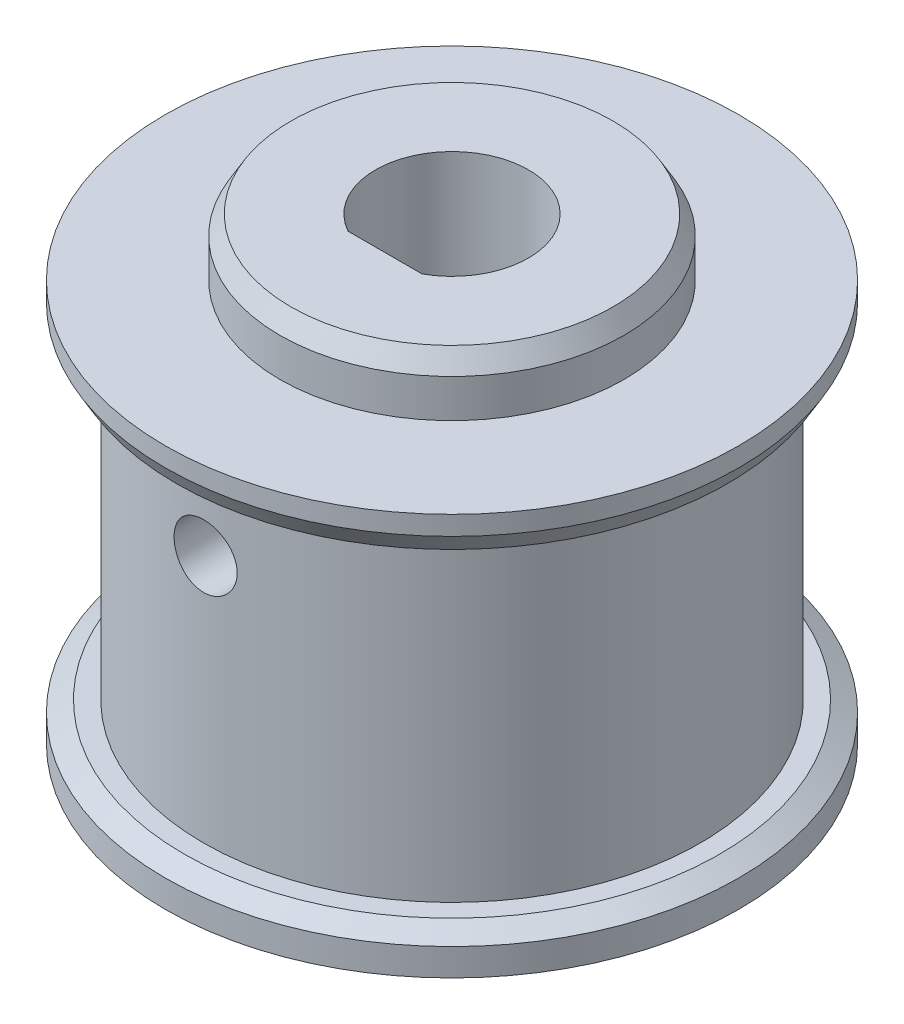
SolidWorks part; units mm, degrees
material "6061 合金"
ref_plane "前视基准面" through (0, 0, 0) normal (0, 0, 1) x (1, 0, 0)
ref_plane "上视基准面" through (0, 0, 0) normal (0, 1, 0) x (1, 0, 0)
ref_plane "右视基准面" through (0, 0, 0) normal (1, 0, 0) x (0, 0, -1)
sketch "草图1" plane through (0, 0, 0) normal (0, 0, 1) x (1, 0, 0)
  line L0 (0, 0) -> (0, 32.2299) construction
  line L1 (4, 0) -> (4, 21)
  line L2 (4, 21) -> (15, 21)
  line L3 (15, 21) -> (15, 19)
  line L4 (15, 19) -> (12.99, 19)
  line L5 (12.99, 19) -> (12.99, 2)
  line L6 (12.99, 2) -> (15, 2)
  line L7 (15, 2) -> (15, 0)
  line L8 (15, 0) -> (4, 0)
  dimension "D1" = 2
  dimension "D2" = 2
  dimension "D3" = 8
  dimension "D4" = 25.98
  dimension "D5" = 30
  dimension "D6" = 21
revolve "旋转1" add sketch "草图1" angle 360 about L0
sketch "草图5" plane through (0, 0, 0) normal (0, -1, 0) x (1, 0, 0)
  circle A0 centre (0, 0) radius 20.5663
extrude "切除-拉伸1" cut sketch "草图5" against normal blind 0.5
sketch "草图6" plane through (0, 21, 0) normal (0, 1, 0) x (1, 0, 0)
  circle A0 centre (0, 0) radius 21.5283
extrude "切除-拉伸2" cut sketch "草图6" against normal blind 0.5
sketch "草图7" plane through (0, 20.5, 0) normal (0, 1, 0) x (1, 0, 0)
  circle A0 centre (0, 0) radius 4 construction
  circle A1 centre (0, 0) radius 4
  circle A2 centre (0, 0) radius 8.5
  dimension "D1" = 17
extrude "凸台-拉伸1" add sketch "草图7" along normal blind 11
sketch "草图10" plane through (0, 20.5, 0) normal (0, 1, 0) x (1, 0, 0)
  circle A1 centre (0, 0) radius 15
  circle A2 centre (0, 0) radius 15
  dimension "D1" = 0
extrude "切除-拉伸3" cut sketch "草图10" along normal blind 15
sketch "草图11" plane through (0, 20.5, 0) normal (0, 1, 0) x (1, 0, 0)
  circle A0 centre (0, 0) radius 4 construction
  circle A1 centre (0, 0) radius 15
  circle A2 centre (0, 0) radius 15
  circle A3 centre (0, 0) radius 4
  dimension "D1" = 0
extrude "凸台-拉伸2" add sketch "草图11" along normal blind 0.5
sketch "草图12" plane through (0, 0.5, 0) normal (0, -1, 0) x (1, 0, 0)
  circle A0 centre (0, 0) radius 4 construction
  circle A1 centre (0, 0) radius 15
  circle A2 centre (0, 0) radius 15
  circle A3 centre (0, 0) radius 4
  dimension "D1" = 0
extrude "凸台-拉伸3" add sketch "草图12" along normal blind 0.5
sketch "草图14" plane through (0, 21, 0) normal (0, 1, 0) x (1, 0, 0)
  circle A0 centre (0, 0) radius 4 construction
  circle A1 centre (0, 0) radius 4
  circle A2 centre (0, 0) radius 7
  dimension "D1" = 14
extrude "凸台-拉伸5" add sketch "草图14" along normal blind 8
sketch "草图17" plane through (0, 21, 0) normal (0, 1, 0) x (1, 0, 0)
  circle A0 centre (0, 0) radius 17.2152
extrude "切除-拉伸4" cut sketch "草图17" along normal through all
sketch "草图18" plane through (0, 21, 0) normal (0, 1, 0) x (1, 0, 0)
  circle A0 centre (0, 0) radius 4 construction
  circle A1 centre (0, 0) radius 4
  circle A2 centre (0, 0) radius 9
  dimension "D1" = 18
extrude "凸台-拉伸6" add sketch "草图18" along normal blind 8
chamfer "倒角1" distance 1 angle 30 1 edges at (0, 19, -15)
chamfer "倒角2" distance 1 angle 30 1 edges at (0, 2, -15)
chamfer "倒角3" distance 0.5 angle 45 1 edges at (0, 29, 9)
sketch "草图21" plane through (0, 29, 0) normal (0, 1, 0) x (1, 0, 0)
  line L0 (-1.9365, -3.5) -> (1.9365, -3.5)
  circle A0 centre (0, 0) radius 4 construction
  arc A1 (-1.9365, -3.5) -> (1.9365, -3.5) centre (0, 0) ccw
  point P5 (0, -4)
  dimension "D1" = 0.5
extrude "凸台-拉伸8" add sketch "草图21" against normal through all
hole_wizard "M4 螺纹孔1" positions "草图20" profile "草图19" tap size "M4" standard "GB"
sketch "草图20" plane through (0, 0, 0) normal (0, 0, 1) x (1, 0, 0)
  line L0 (4, 29) -> (-4, 29) construction
  point P0 (0, 15)
  dimension "D1" = 14
sketch "草图19" plane through (0, 15, 0) normal (1, 0, 0) x (0, 1, 0)
  line L0 (0, 0) -> (0, 15)
  line L1 (0, 15) -> (1.65, 15)
  line L2 (1.65, 15) -> (1.65, 0)
  line L5 (1.65, 0) -> (0, 0)
  line L11 (0, -6.35) -> (0, 107.95) construction
  dimension "通孔螺纹孔钻头直径" = 3.3
  dimension "通孔螺纹孔钻头深度" = 15
cosmetic thread "孔螺蚊线1" parameters "D2"=4
pattern_circular "阵列(圆周)1" count 2 every 90 of "M4 螺纹孔1"
sketch "草图22" plane through (0, 29, 0) normal (0, 1, 0) x (1, 0, 0)
  circle A0 centre (0, 0) radius 11.2279
extrude "切除-拉伸5" cut sketch "草图22" against normal blind 5
chamfer "倒角4" distance 1 angle 30 1 edges at (0, 24, 9)
